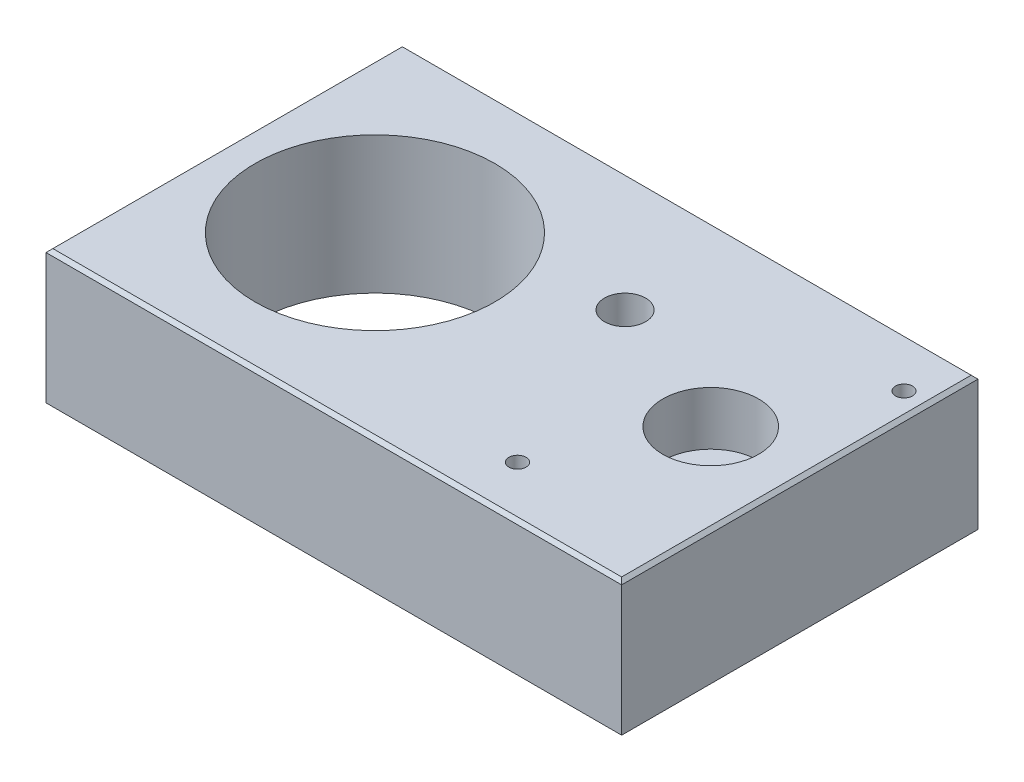
SolidWorks part; units mm, degrees
ref_plane "Front Plane" through (0, 0, 0) normal (0, 0, 1) x (1, 0, 0)
ref_plane "Top Plane" through (0, 0, 0) normal (0, 1, 0) x (1, 0, 0)
ref_plane "Right Plane" through (0, 0, 0) normal (1, 0, 0) x (0, 0, -1)
sketch "Sketch1" plane through (0, 0, 0) normal (0, 1, 0) x (1, 0, 0)
  line L1 (-42, 26) -> (42, 26)
  line L2 (-42, 26) -> (-42, -26)
  line L3 (-42, -26) -> (42, -26)
  line L4 (42, 26) -> (42, -26)
  line L5 (-42, 26) -> (42, -26) construction
  line L6 (-42, -26) -> (42, 26) construction
  point P0 (0, 0)
  dimension "D1" = 52
  dimension "D2" = 84
extrude "Boss-Extrude1" add sketch "Sketch1" along normal blind 20
sketch "Sketch2" plane through (0, 20, 0) normal (0, 1, 0) x (1, 0, 0)
  line L0 (-42, 26) -> (-42, -26) construction
  circle A0 centre (-20, 0) radius 17.5
  dimension "D1" = 35
  dimension "D2" = 22
extrude "Cut-Extrude1" cut sketch "Sketch2" against normal blind 20
sketch "Sketch3" plane through (0, 20, 0) normal (0, 1, 0) x (1, 0, 0)
  line L0 (-42, 26) -> (-42, -26) construction
  line L1 (42, 26) -> (-42, 26) construction
  circle A0 centre (8, 8.5) radius 3
  dimension "D1" = 6
  dimension "D2" = 50
  dimension "D3" = 17.5
extrude "Cut-Extrude2" cut sketch "Sketch3" against normal blind 20
sketch "Sketch4" plane through (0, 20, 0) normal (0, 1, 0) x (1, 0, 0)
  line L0 (42, -26) -> (42, 26) construction
  line L1 (-42, -26) -> (42, -26) construction
  line L2 (42, 26) -> (-42, 26) construction
  circle A0 centre (19.4, -18.6) radius 1.25
  circle A1 centre (38.6, 18.6) radius 1.25
  dimension "D1" = 2.5
  dimension "D2" = 2.5
  dimension "D3" = 22.6
  dimension "D4" = 7.4
  dimension "D5" = 7.4
  dimension "D6" = 3.4
extrude "Cut-Extrude3" cut sketch "Sketch4" against normal blind 20 contours A0 | A1
sketch "Sketch5" plane through (0, 20, 0) normal (0, 1, 0) x (1, 0, 0)
  line L0 (-42, 26) -> (-42, -26) construction
  circle A0 centre (29, 0) radius 4
  dimension "D1" = 8
  dimension "D2" = 71
extrude "Cut-Extrude4" cut sketch "Sketch5" against normal blind 20 contours A0
sketch "Sketch6" plane through (0, 20, 0) normal (0, 1, 0) x (1, 0, 0)
  circle A0 centre (29, 0) radius 7
  dimension "D1" = 14
extrude "Cut-Extrude5" cut sketch "Sketch6" against normal blind 7.8
chamfer "Chamfer1" distance 0.5 angle 45 8 edges at (42, 20, 0) (0, 20, 26) (-42, 20, 0) (0, 20, -26) (0, 0, -26) (42, 0, 0) (-42, 0, 0) (0, 0, 26)
